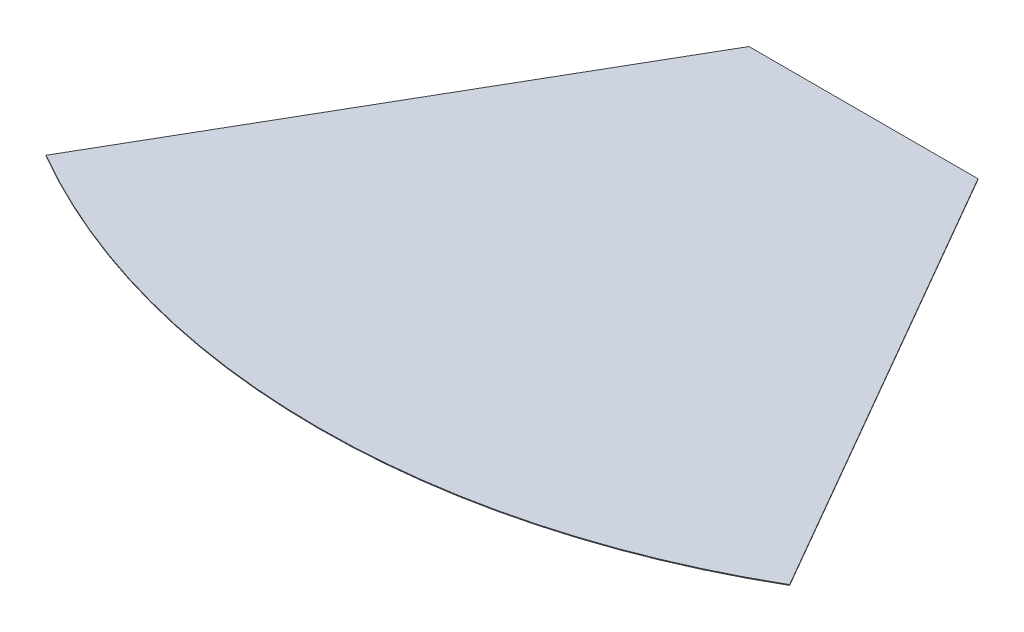
SolidWorks part; units mm, degrees
material "Aluminum alloy plate"
ref_plane "Front Plane" through (0, 0, 0) normal (0, 0, 1) x (1, 0, 0)
ref_plane "Top Plane" through (0, 0, 0) normal (0, 1, 0) x (1, 0, 0)
ref_plane "Right Plane" through (0, 0, 0) normal (1, 0, 0) x (0, 0, -1)
sketch "Sketch1" plane through (0, 0, 0) normal (0, 1, 0) x (1, 0, 0)
  line L0 (-462, 0) -> (462, 0)
  line L1 (462, 0) -> (1500, -1797.8687)
  line L2 (0, 0) -> (0, -1319.0559) construction
  line L3 (-462, 0) -> (-1500, -1797.8687)
  arc A0 (-1500, -1797.8687) -> (1500, -1797.8687) centre (0, 800.2075) ccw
  dimension "D1" = 924
  dimension "D4" = 3000
  dimension "D2" = 2076
  dimension "D3" = 3000
extrude "Boss-Extrude1" add sketch "Sketch1" along normal blind 3
